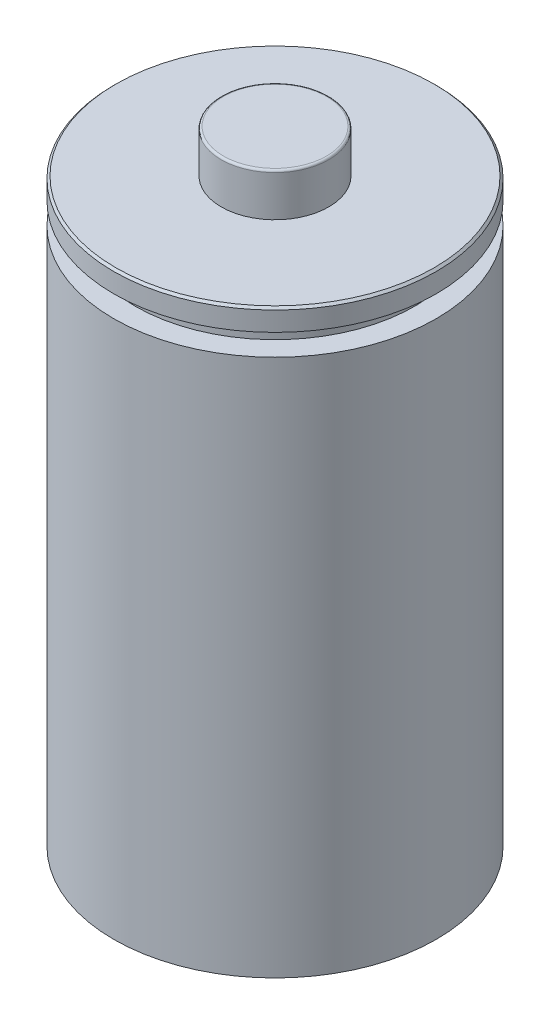
SolidWorks part; units mm, degrees
ref_plane "Front Plane" through (0, 0, 0) normal (0, 0, 1) x (1, 0, 0)
ref_plane "Top Plane" through (0, 0, 0) normal (0, 1, 0) x (1, 0, 0)
ref_plane "Right Plane" through (0, 0, 0) normal (1, 0, 0) x (0, 0, -1)
other "Configuration Table"
sketch "Sketch1" plane through (0, 0, 0) normal (0, 1, 0) x (1, 0, 0)
  circle A0 centre (0, 0) radius 75
  dimension "D1" = 150
extrude "Boss-Extrude1" add sketch "Sketch1" along normal blind 250 contours A0
sketch "Sketch2" plane through (0, 250, 0) normal (0, 1, 0) x (1, 0, 0)
  circle A0 centre (0, 0) radius 65
  dimension "D1" = 130
extrude "Boss-Extrude2" add sketch "Sketch2" along normal blind 10 contours A0
sketch "Sketch3" plane through (0, 260, 0) normal (0, 1, 0) x (1, 0, 0)
  circle A0 centre (0, 0) radius 75 construction
  circle A1 centre (0, 0) radius 75
extrude "Boss-Extrude3" add sketch "Sketch3" along normal blind 10 contours A1
sketch "Sketch4" plane through (0, 270, 0) normal (0, 1, 0) x (1, 0, 0)
  circle A0 centre (0, 0) radius 25
  dimension "D1" = 50
extrude "Boss-Extrude4" add sketch "Sketch4" along normal blind 20 contours A0
fillet "Fillet1" radius 1 1 edges at (0, 290, 25)
chamfer "Chamfer1" distance 1 angle 45 1 edges at (0, 270, 75)
